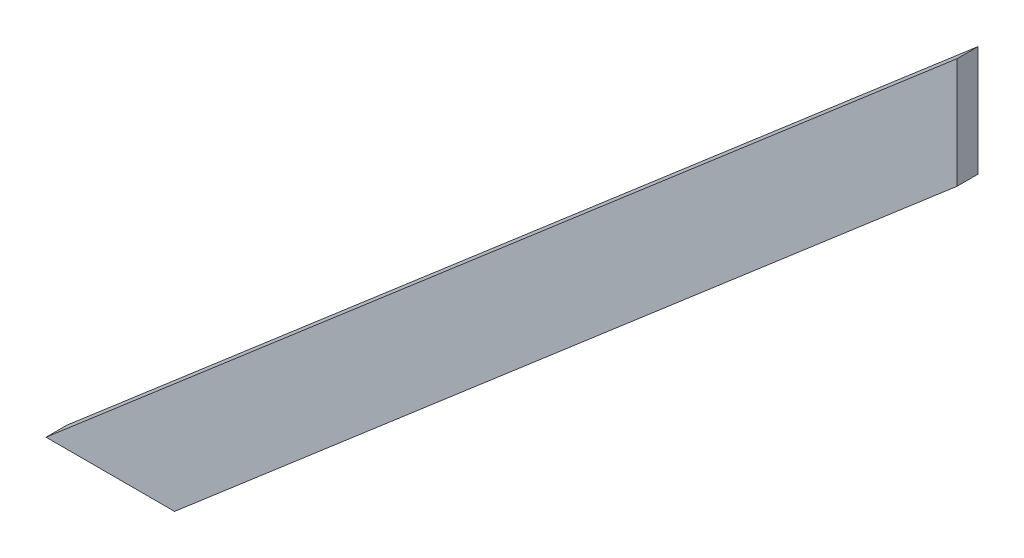
from build123d import *

# Parameters (mm, degrees)
BOSS_EXTRUDE1_DEPTH = 50


with BuildPart() as part:
    # Sketch1 → Boss-Extrude1 (new body)
    with BuildSketch(Plane.XY):
        Polygon((-1213.383462756, 12946.407177591), (-906.620260802, 12946.407177591), (960.48224113, 14551.812970124), (960.48224113, 14815.579646482), align=None)
    extrude(amount=BOSS_EXTRUDE1_DEPTH)


solid = part.part
